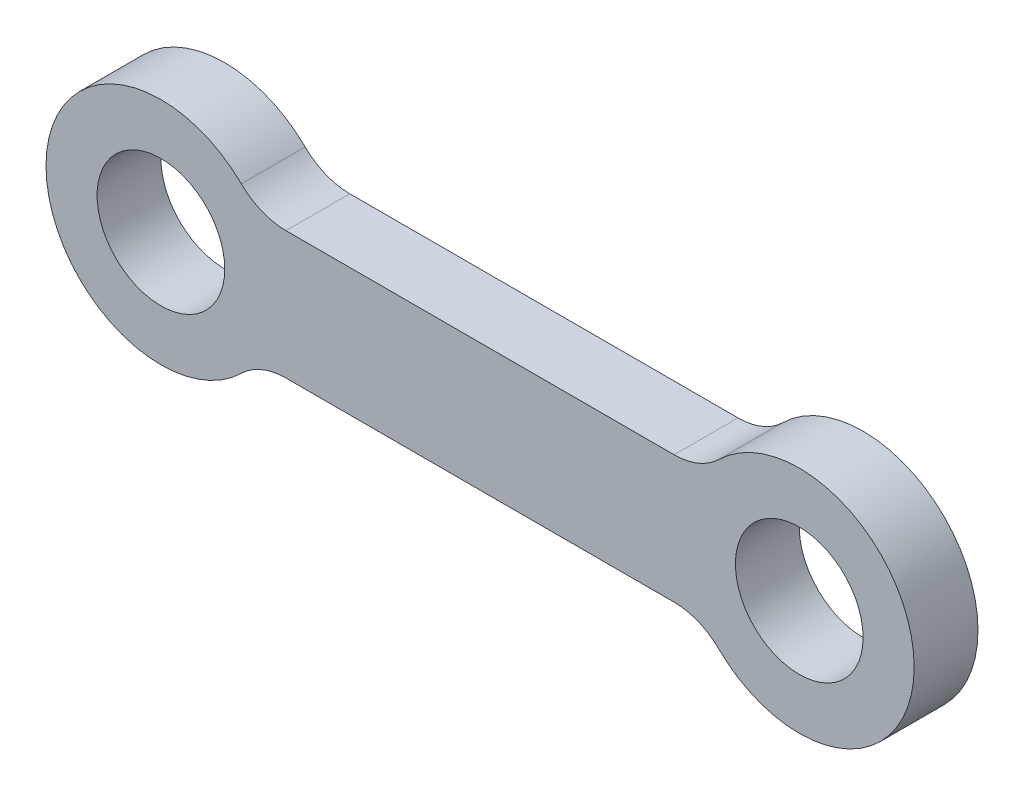
from build123d import *

# Parameters (mm, degrees)
SKETCH1_R           = 5
BOSS_EXTRUDE1_DEPTH = 5


with BuildPart() as part:
    # Sketch1 → Boss-Extrude1 (new body)
    with BuildSketch(Plane.XY):
        with BuildLine():
            Line((9.797958971, 5), (40.202041029, 5))
            ThreePointArc((40.202041029, 5), (42.091863394, 5.370899501), (43.70131209, 6.428571429))
            ThreePointArc((43.70131209, 6.428571429), (59, 0), (43.70131209, -6.428571429))
            ThreePointArc((43.70131209, -6.428571429), (42.091863394, -5.370899501), (40.202041029, -5))
            Line((40.202041029, -5), (9.797958971, -5))
            ThreePointArc((9.797958971, -5), (7.908136606, -5.370899501), (6.29868791, -6.428571429))
            ThreePointArc((6.29868791, -6.428571429), (-9, 0), (6.29868791, 6.428571429))
            ThreePointArc((6.29868791, 6.428571429), (7.908136606, 5.370899501), (9.797958971, 5))
        make_face()
        Circle(SKETCH1_R, mode=Mode.SUBTRACT)
        with Locations((50, 0)):
            Circle(SKETCH1_R, mode=Mode.SUBTRACT)
    extrude(amount=BOSS_EXTRUDE1_DEPTH)


solid = part.part
